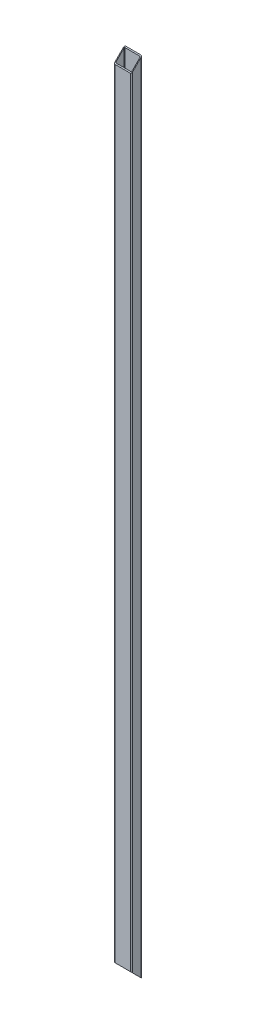
from build123d import *

# Parameters (mm, degrees)
BOSS_EXTRUDE1_DEPTH     = 2270
CUT_EXTRUDE1_DEPTH      = 2271.600140932
CUT_EXTRUDE1_DEPTH_BACK = 2271.600140932


with BuildPart() as part:
    # Sketch1 → Boss-Extrude1 (new body)
    with BuildSketch(Plane(origin=(0, 0, 0), x_dir=(1, 0, 0), z_dir=(0, 1, 0))):
        with BuildLine():
            Line((-21.55, -15), (21.55, -15))
            ThreePointArc((21.55, -15), (23.989518395, -13.989518395), (25, -11.55))
            Line((25, -11.55), (25, 11.55))
            ThreePointArc((25, 11.55), (23.989518395, 13.989518395), (21.55, 15))
            Line((21.55, 15), (-21.55, 15))
            ThreePointArc((-21.55, 15), (-23.989518395, 13.989518395), (-25, 11.55))
            Line((-25, 11.55), (-25, -11.55))
            ThreePointArc((-25, -11.55), (-23.989518395, -13.989518395), (-21.55, -15))
        make_face()
        with BuildLine():
            Line((-21.55, -12.7), (21.55, -12.7))
            ThreePointArc((21.55, -12.7), (22.363172798, -12.363172798), (22.7, -11.55))
            Line((22.7, -11.55), (22.7, 11.55))
            ThreePointArc((22.7, 11.55), (22.363172798, 12.363172798), (21.55, 12.7))
            Line((21.55, 12.7), (-21.55, 12.7))
            ThreePointArc((-21.55, 12.7), (-22.363172798, 12.363172798), (-22.7, 11.55))
            Line((-22.7, 11.55), (-22.7, -11.55))
            ThreePointArc((-22.7, -11.55), (-22.363172798, -12.363172798), (-21.55, -12.7))
        make_face(mode=Mode.SUBTRACT)
    extrude(amount=BOSS_EXTRUDE1_DEPTH)

    # Sketch2 → Cut-Extrude1 (cut, two sides: drawn at the far end of the back side and taken through both)
    with BuildSketch(Plane(origin=(25, 0, 0), x_dir=(0, 0, -1), z_dir=(1, 0, 0)).offset(-CUT_EXTRUDE1_DEPTH_BACK)):
        Polygon((15, 2270), (-15, 2240), (-15, 2270), align=None)
        Polygon((15, 0), (-15, 0), (-15, 30), align=None)
    extrude(amount=CUT_EXTRUDE1_DEPTH + CUT_EXTRUDE1_DEPTH_BACK, mode=Mode.SUBTRACT)


solid = part.part
